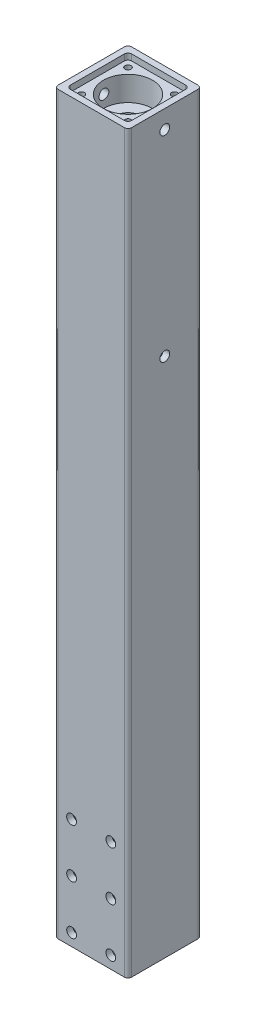
SolidWorks part; units mm, degrees
ref_plane "Front Plane" through (0, 0, 0) normal (0, 0, 1) x (1, 0, 0)
ref_plane "Top Plane" through (0, 0, 0) normal (0, 1, 0) x (1, 0, 0)
ref_plane "Right Plane" through (0, 0, 0) normal (1, 0, 0) x (0, 0, -1)
other "Configuration Table"
sketch "Sketch1" plane through (0, 0, 0) normal (0, 1, 0) x (1, 0, 0)
  line L1 (-30, 30) -> (30, 30)
  line L2 (-30, 30) -> (-30, -30)
  line L3 (-30, -30) -> (30, -30)
  line L4 (30, 30) -> (30, -30)
  line L5 (-30, 30) -> (30, -30) construction
  line L6 (-30, -30) -> (30, 30) construction
  point P0 (0, 0)
  dimension "D1" = 60
  dimension "D2" = 60
extrude "Boss-Extrude1" add sketch "Sketch1" along normal blind 600
sketch "Sketch2" plane through (0, 600, 0) normal (0, 1, 0) x (1, 0, 0)
  line L1 (-25, 25) -> (25, 25)
  line L2 (-25, 25) -> (-25, -25)
  line L3 (-25, -25) -> (25, -25)
  line L4 (25, 25) -> (25, -25)
  line L5 (-25, 25) -> (25, -25) construction
  line L6 (-25, -25) -> (25, 25) construction
  point P0 (0, 0)
  dimension "D1" = 50
  dimension "D2" = 50
extrude "Cut-Extrude1" cut sketch "Sketch2" against normal blind 5
sketch "Sketch3" plane through (0, 595, 0) normal (0, 1, 0) x (1, 0, 0)
  circle A0 centre (0, 0) radius 20
  dimension "D1" = 40
sketch "Sketch4" plane through (0, 0, 0) normal (1, 0, 0) x (0, 0, -1)
  circle A0 centre (0, 585) radius 4
  dimension "D2" = 8
extrude "Cut-Extrude3" cut sketch "Sketch4" against normal blind 30 and the other way blind 600
fillet "Fillet2" radius 3 4 edges at (30, 300, -30) (-30, 300, -30) (-30, 300, 30) (30, 300, 30)
extrude "Cut-Extrude4" cut sketch "Sketch3" against normal blind 20
sketch "Sketch5" plane through (0, 0, 0) normal (0, -1, 0) x (1, 0, 0)
  line L1 (-25, 25) -> (25, 25)
  line L2 (-25, 25) -> (-25, -25)
  line L3 (-25, -25) -> (25, -25)
  line L4 (25, 25) -> (25, -25)
  line L5 (-25, 25) -> (25, -25) construction
  line L6 (-25, -25) -> (25, 25) construction
  point P0 (0, 0)
  dimension "D1" = 50
  dimension "D2" = 50
extrude "Cut-Extrude5" cut sketch "Sketch5" against normal blind 110
sketch "Sketch6" plane through (0, 110, 0) normal (0, -1, 0) x (1, 0, 0)
  circle A0 centre (0, 0) radius 25
  dimension "D1" = 50
extrude "Cut-Extrude6" cut sketch "Sketch6" against normal blind 450
sketch "Sketch7" plane through (0, 575, 0) normal (0, 1, 0) x (1, 0, 0)
  circle A0 centre (0, 0) radius 10
  dimension "D1" = 20
extrude "Cut-Extrude7" cut sketch "Sketch7" against normal blind 15
fillet "Fillet4" radius 3 4 edges at (25, 597.5, 25) (-25, 597.5, 25) (25, 597.5, -25) (-25, 597.5, -25)
sketch "Sketch8" plane through (0, 0, 0) normal (1, 0, 0) x (0, 0, -1)
  circle A0 centre (0, 425) radius 4
  dimension "D2" = 8
extrude "Cut-Extrude8" cut sketch "Sketch8" against normal blind 30 and the other way blind 30
sketch "Sketch9" plane through (0, 0, 0) normal (0, 0, 1) x (1, 0, 0)
  line L0 (0, 0) -> (0, 50)
  circle A0 centre (-16, 10) radius 4
  circle A1 centre (-16, 50) radius 4
  circle A2 centre (-16, 90) radius 4
  circle A3 centre (16, 10) radius 4
  circle A4 centre (16, 90) radius 4
  circle A5 centre (16, 50) radius 4
  dimension "D4" = 8
  dimension "D5" = 8
  dimension "D6" = 8
  dimension "D2" = 80
  dimension "D3" = 32
extrude "Cut-Extrude9" cut sketch "Sketch9" against normal blind 30 and the other way blind 30 contours A1 | A4 | A5 | A2 | A3 | A0
sketch "Sketch10" plane through (0, 595, 0) normal (0, 1, 0) x (1, 0, 0)
  circle A0 centre (-19, 19) radius 2.5
  circle A1 centre (19, 19) radius 2.5
  circle A2 centre (19, -19) radius 2.5
  circle A3 centre (-19, -19) radius 2.5
  point P0 (0, 0)
  dimension "D3" = 5
  dimension "D4" = 5
  dimension "D5" = 5
  dimension "D6" = 5
  dimension "D1" = 38
  dimension "D2" = 38
extrude "Cut-Extrude10" cut sketch "Sketch10" against normal blind 20
